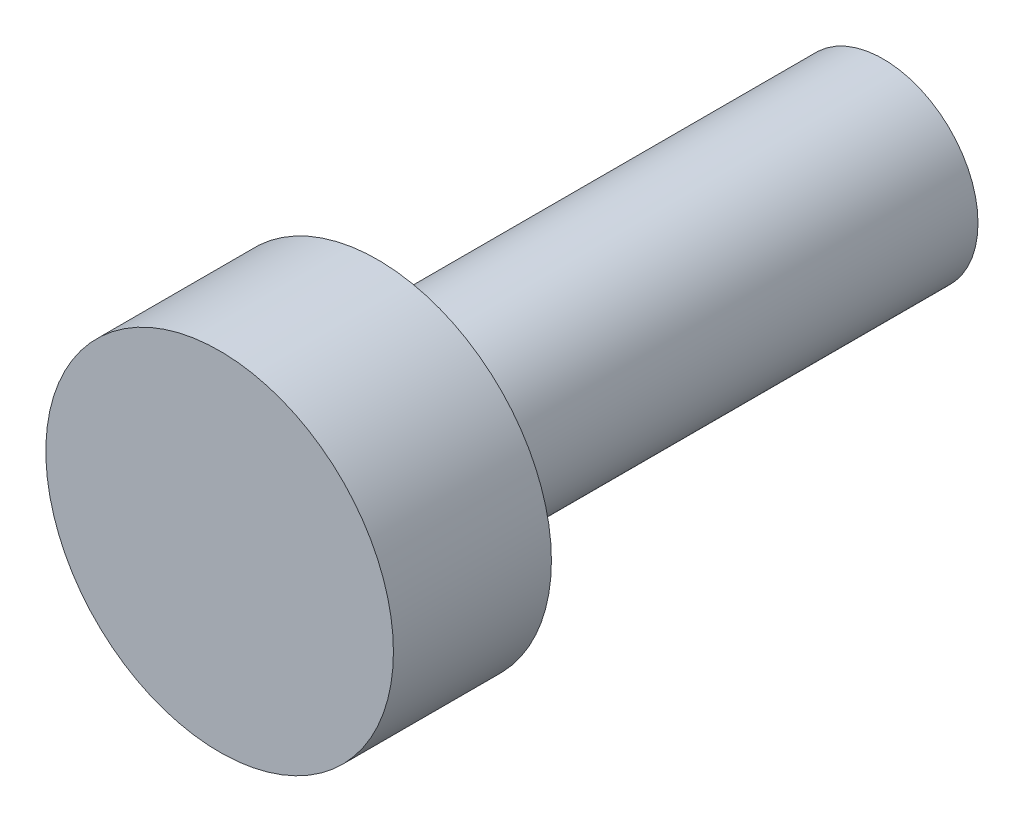
from build123d import *

# Parameters (mm, degrees)
SKETCH_1_R      = 1.5
EXTRUDE_1_DEPTH = 8
SKETCH_2_R      = 2.75
EXTRUDE_2_DEPTH = 2.5


with BuildPart() as part:
    # 草图1 → 凸台-拉伸1 (new body)
    with BuildSketch(Plane.XY):
        Circle(SKETCH_1_R)
    extrude(amount=-EXTRUDE_1_DEPTH)

    # 草图2 → 凸台-拉伸2 (add)
    with BuildSketch(Plane.XY):
        Circle(SKETCH_2_R)
    extrude(amount=EXTRUDE_2_DEPTH)


solid = part.part
